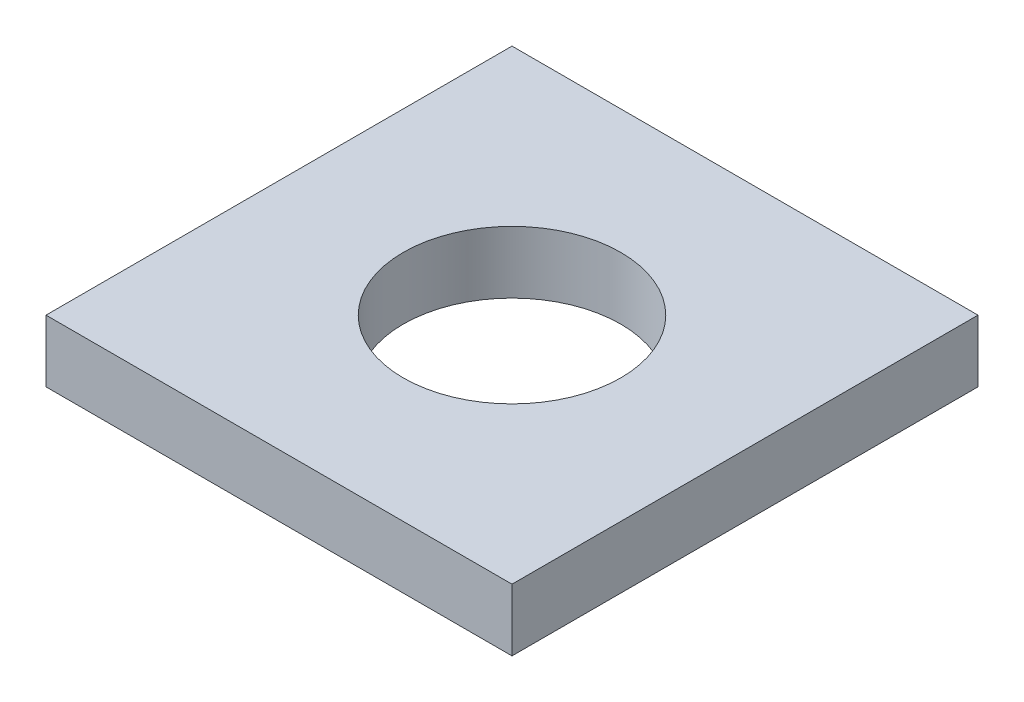
SolidWorks part; units mm, degrees
material "Q235"
ref_plane "Front Plane" through (0, 0, 0) normal (0, 0, 1) x (1, 0, 0)
ref_plane "Top Plane" through (0, 0, 0) normal (0, 1, 0) x (1, 0, 0)
ref_plane "Right Plane" through (0, 0, 0) normal (1, 0, 0) x (0, 0, -1)
sketch "Sketch1" plane through (0, 0, 0) normal (0, 1, 0) x (1, 0, 0)
  line L1 (0, 0) -> (30, 0)
  line L2 (0, 0) -> (0, -30)
  line L3 (0, -30) -> (30, -30)
  line L4 (30, 0) -> (30, -30)
  dimension "D1" = 30
  dimension "D2" = 30
extrude "Boss-Extrude1" add sketch "Sketch1" along normal blind 4
sketch "Sketch3" plane through (0, 4, 0) normal (0, 1, 0) x (1, 0, 0)
  line L0 (0, -15) -> (15, -15) construction
  line L1 (0, 0) -> (0, -30) construction
  circle A0 centre (15, -15) radius 7
  dimension "D1" = 14
  dimension "D2" = 15
extrude "Cut-Extrude2" cut sketch "Sketch3" against normal through all
sketch "Sketch4" plane through (0, 4, 0) normal (0, 1, 0) x (1, 0, 0)
  line L0 (0, -30) -> (30, -30) construction
  line L1 (0, 0) -> (50, 0)
  line L2 (0, 0) -> (0, -30)
  line L3 (0, -30) -> (50, -30)
  line L4 (50, 0) -> (50, -30)
  dimension "D1" = 50
extrude "Cut-Extrude3" [suppressed] cut sketch "Sketch4" against normal through all
